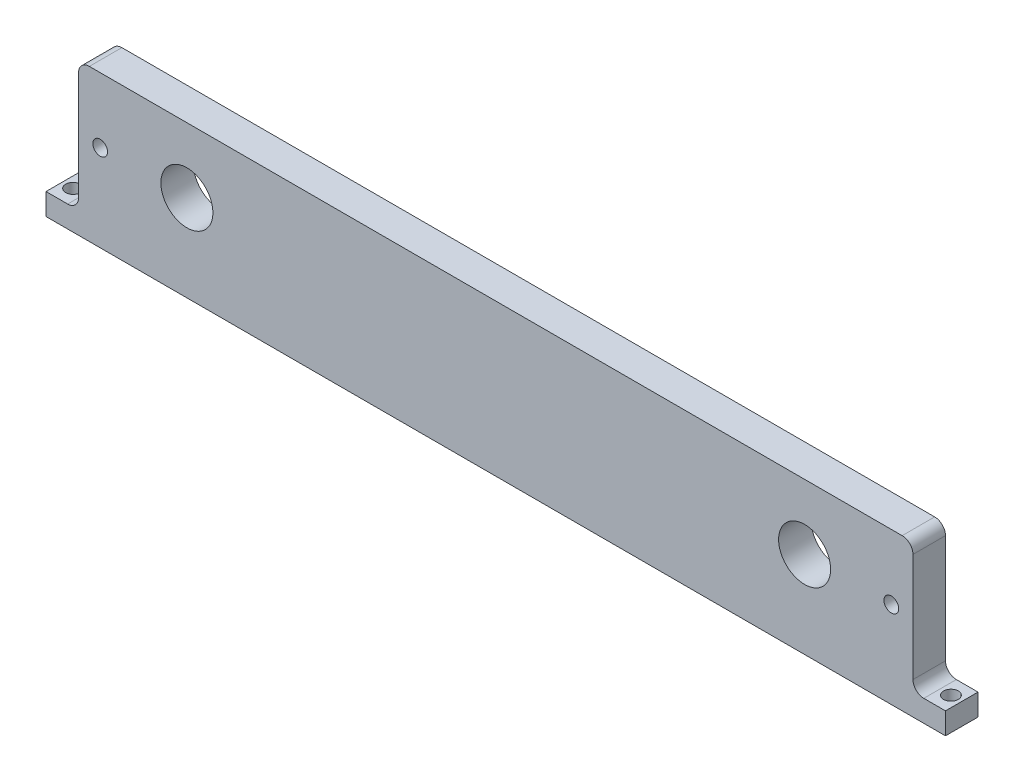
from build123d import *

# Parameters (mm, degrees)
SKETCH1_W                      = 415
SKETCH1_H                      = 70
BOSS_EXTRUDE1_DEPTH            = 15
SKETCH2_R                      = 3.4
SKETCH2_R_2                    = 12
CUT_EXTRUDE1_DEPTH             = 211.965044498
SKETCH10_W                     = 15
SKETCH10_H                     = 60
CUT_EXTRUDE2_DEPTH             = 211.965044498
F_6_8_6_8_DIAMETER_HOLE1_D     = 6.8
F_6_8_6_8_DIAMETER_HOLE1_DEPTH = 12.4
F_6_8_6_8_DIAMETER_HOLE1_TIP   = 2.042926105
FILLET1_R                      = 5
FILLET2_R                      = 5
M6_TAPPED_HOLE1_D              = 5
M6_TAPPED_HOLE1_DEPTH          = 15
M6_TAPPED_HOLE1_TIP            = 1.502151548


with BuildPart() as part:
    # Sketch1 → Boss-Extrude1 (new body)
    with BuildSketch(Plane.XY):
        Rectangle(SKETCH1_W, SKETCH1_H)
    extrude(amount=BOSS_EXTRUDE1_DEPTH)

    # Sketch2 → Cut-Extrude1 (cut, through all)
    with BuildSketch(Plane.XY.offset(15)):
        with Locations((-182.5, 5)):
            Circle(SKETCH2_R)
        with Locations((-142.5, 5)):
            Circle(SKETCH2_R_2)
        with Locations((142.5, 5)):
            Circle(SKETCH2_R_2)
        with Locations((182.5, 5)):
            Circle(SKETCH2_R)
    extrude(amount=-CUT_EXTRUDE1_DEPTH, mode=Mode.SUBTRACT)

    # Sketch10 → Cut-Extrude2 (cut, through all)
    with BuildSketch(Plane.XY.offset(15)):
        with Locations((-200, 5)):
            Rectangle(SKETCH10_W, SKETCH10_H)
        with Locations((200, 5)):
            Rectangle(SKETCH10_W, SKETCH10_H)
    extrude(amount=-CUT_EXTRUDE2_DEPTH, mode=Mode.SUBTRACT)

    # Ø6.8 (6.8) Diameter Hole1
    with Locations(Plane(origin=(0, -35, 0), x_dir=(-1, 0, 0), z_dir=(0, -1, 0))):
        with Locations((-202.5, -7.5), (202.5, -7.5)):
            Hole(F_6_8_6_8_DIAMETER_HOLE1_D / 2, depth=F_6_8_6_8_DIAMETER_HOLE1_DEPTH)
            with Locations((0, 0, -(F_6_8_6_8_DIAMETER_HOLE1_DEPTH + F_6_8_6_8_DIAMETER_HOLE1_TIP / 2))):  # 118° drill point
                Cone(0, F_6_8_6_8_DIAMETER_HOLE1_D / 2, F_6_8_6_8_DIAMETER_HOLE1_TIP, mode=Mode.SUBTRACT)

    # Fillet1
    fillet1_edges = [part.edges().sort_by_distance(p)[0] for p in [
        (-192.5, -25, 7.5),
        (192.5, -25, 7.5),
    ]]
    fillet(fillet1_edges, radius=FILLET1_R)

    # Fillet2
    fillet2_edges = [part.edges().sort_by_distance(p)[0] for p in [
        (-192.5, 35, 7.5),
        (192.5, 35, 7.5),
    ]]
    fillet(fillet2_edges, radius=FILLET2_R)

    # M6 Tapped Hole1
    with Locations(Plane(origin=(0, -35, 0), x_dir=(-1, 0, 0), z_dir=(0, -1, 0))):
        with Locations((125, -7.5), (-125, -7.5)):
            Hole(M6_TAPPED_HOLE1_D / 2, depth=M6_TAPPED_HOLE1_DEPTH)
            with Locations((0, 0, -(M6_TAPPED_HOLE1_DEPTH + M6_TAPPED_HOLE1_TIP / 2))):  # 118° drill point
                Cone(0, M6_TAPPED_HOLE1_D / 2, M6_TAPPED_HOLE1_TIP, mode=Mode.SUBTRACT)


solid = part.part
